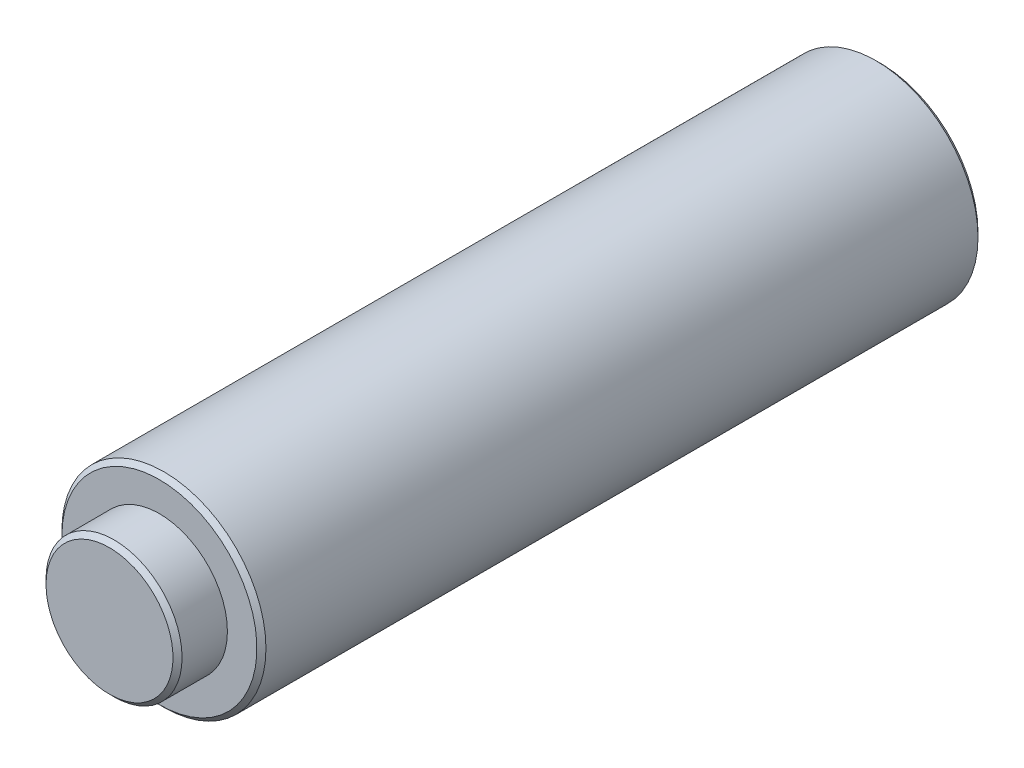
from build123d import *

# Parameters (mm, degrees)
CHAMFER1_SIZE = 1


with BuildPart() as part:
    # Sketch1 → Revolve1 (revolve)
    with BuildSketch(Plane(origin=(0, 0, 0), x_dir=(0, 0, -1), z_dir=(1, 0, 0)), mode=Mode.PRIVATE) as revolve1_sk:
        Polygon((178, 0), (178, 9), (170, 9), (170, 22.5), (11, 22.5), (11, 15), (0, 15), (0, 0), align=None)
    revolve(revolve1_sk.sketch.rotate(Axis((0, 0, 0), (0, 0, -1)), 90), axis=Axis((0, 0, 0), (0, 0, -1)))

    # Chamfer1
    chamfer1_edges = [part.edges().sort_by_distance(p)[0] for p in [
        (-15, 0, 0),
        (-22.5, 0, -11),
        (-22.5, 0, -170),
        (-9, 0, -178),
    ]]
    chamfer(chamfer1_edges, length=CHAMFER1_SIZE)


solid = part.part
